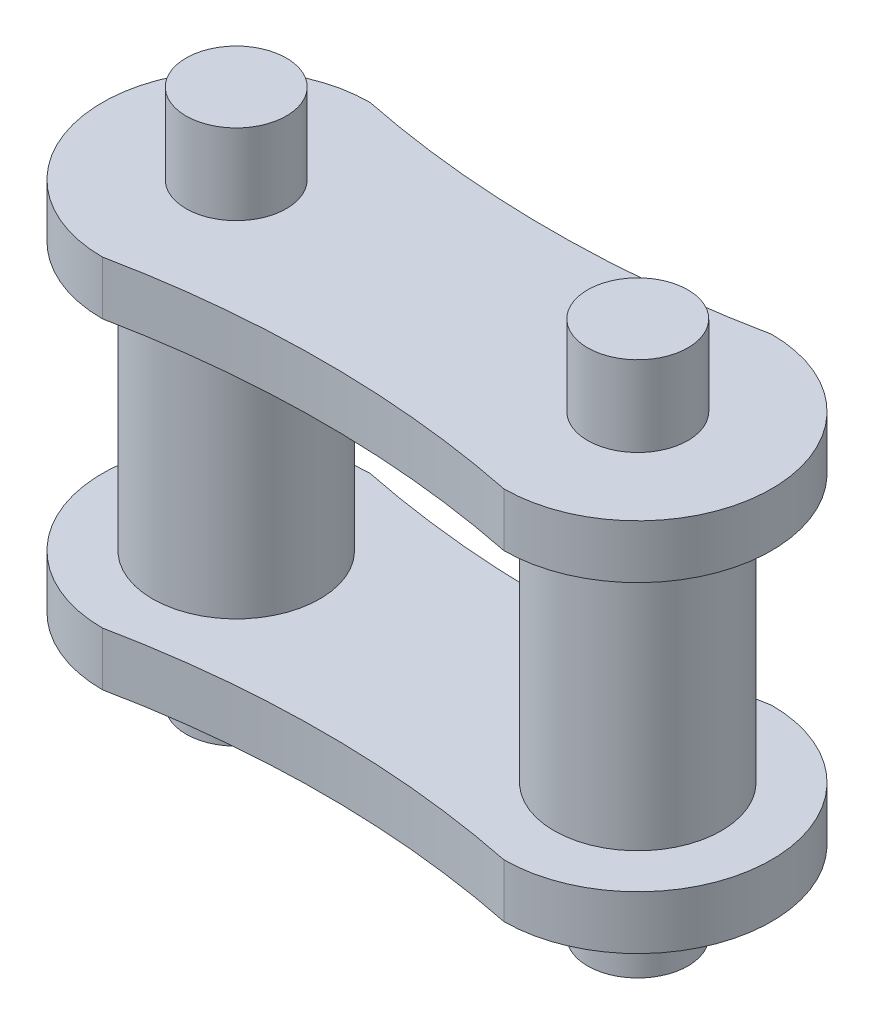
from build123d import *

# Parameters (mm, degrees)
BOSS_EXTRUDE1_DEPTH = 8
SKETCH2_R           = 12.5
BOSS_EXTRUDE2_DEPTH = 40
LPATTERN1_COUNT     = 2
LPATTERN1_PITCH     = 48
SKETCH3_R           = 7.5
BOSS_EXTRUDE3_DEPTH = 12
LPATTERN2_COUNT     = 2
LPATTERN2_PITCH     = 68


with BuildPart() as part:
    # Sketch1 → Boss-Extrude1 (new body)
    with BuildSketch(Plane(origin=(0, 0, 0), x_dir=(1, 0, 0), z_dir=(0, 1, 0))):
        with BuildLine():
            ThreePointArc((0, 20), (-20, 0), (0, -20))
            ThreePointArc((0, -20), (30, -16.969384567), (60, -20))
            ThreePointArc((60, -20), (80, 0), (60, 20))
            ThreePointArc((60, 20), (30, 16.969384567), (0, 20))
        make_face()
    boss_extrude1 = extrude(amount=BOSS_EXTRUDE1_DEPTH)

    # Sketch2 → Boss-Extrude2 (add)
    with BuildSketch(Plane(origin=(0, 8, 0), x_dir=(1, 0, 0), z_dir=(0, 1, 0))):
        with Locations(Location((0, 0, 0), (0, 0, 270))):
            Circle(SKETCH2_R)
        with Locations(Location((60, 0, 0), (0, 0, 270))):
            Circle(SKETCH2_R)
    extrude(amount=BOSS_EXTRUDE2_DEPTH)

    # LPattern1: Boss-Extrude1 ×2
    with Locations(*[(0, i * LPATTERN1_PITCH, 0) for i in range(1, LPATTERN1_COUNT)]):
        add(boss_extrude1)

    # Sketch3 → Boss-Extrude3 (add)
    with BuildSketch(Plane(origin=(0, 56, 0), x_dir=(1, 0, 0), z_dir=(0, 1, 0))):
        with Locations(Location((0, 0, 0), (0, 0, 270))):
            Circle(SKETCH3_R)
        with Locations(Location((60, 0, 0), (0, 0, 270))):
            Circle(SKETCH3_R)
    boss_extrude3 = extrude(amount=BOSS_EXTRUDE3_DEPTH)

    # LPattern2: Boss-Extrude3 ×2
    with Locations(*[(0, -i * LPATTERN2_PITCH, 0) for i in range(1, LPATTERN2_COUNT)]):
        add(boss_extrude3)


solid = part.part
